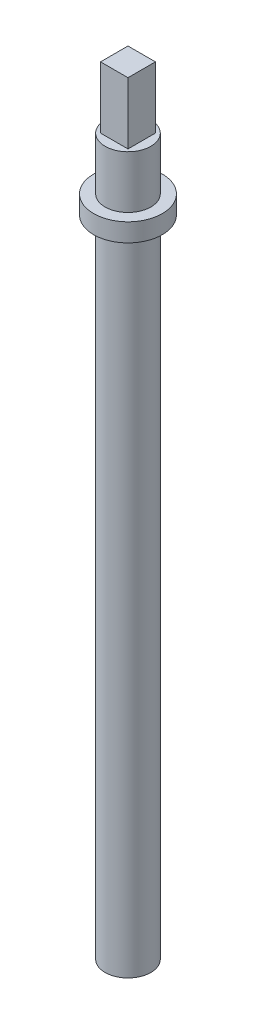
from build123d import *

# Parameters (mm, degrees)
SKETCH1_R           = 10
BOSS_EXTRUDE1_DEPTH = 340
SKETCH2_OUTSIDE_W   = 90.234
SKETCH2_OUTSIDE_H   = 90.234
SKETCH2_OUTSIDE_W_2 = 12
SKETCH2_OUTSIDE_H_2 = 12
CUT_EXTRUDE1_DEPTH  = 27
SKETCH3_R           = 15
BOSS_EXTRUDE2_DEPTH = 8


with BuildPart() as part:
    # Sketch1 → Boss-Extrude1 (new body)
    with BuildSketch(Plane(origin=(0, 0, 0), x_dir=(1, 0, 0), z_dir=(0, 1, 0))):
        with Locations(Location((0, 0, 0), (0, 0, 270))):
            Circle(SKETCH1_R)
    extrude(amount=BOSS_EXTRUDE1_DEPTH)

    # Sketch2 outside → Cut-Extrude1 (cut)
    with BuildSketch(Plane(origin=(0, 340, 0), x_dir=(1, 0, 0), z_dir=(0, 1, 0))):
        Rectangle(SKETCH2_OUTSIDE_W, SKETCH2_OUTSIDE_H)
        Rectangle(SKETCH2_OUTSIDE_W_2, SKETCH2_OUTSIDE_H_2, mode=Mode.SUBTRACT)
    extrude(amount=-CUT_EXTRUDE1_DEPTH, mode=Mode.SUBTRACT)

    # Sketch3 → Boss-Extrude2 (add)
    with BuildSketch(Plane(origin=(0, 282, 0), x_dir=(1, 0, 0), z_dir=(0, 1, 0))):
        with Locations(Location((0, 0, 0), (0, 0, 270))):
            Circle(SKETCH3_R)
    extrude(amount=BOSS_EXTRUDE2_DEPTH)


solid = part.part
